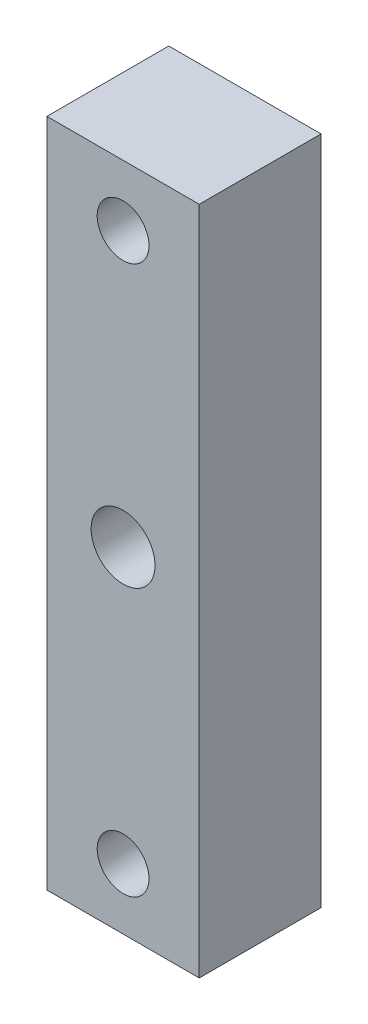
from build123d import *

# Parameters (mm, degrees)
SKETCH1_W                   = 25
SKETCH1_H                   = 110
BOSS_EXTRUDE1_DEPTH         = 20
SKETCH3_R                   = 4.25
CUT_EXTRUDE1_DEPTH          = 30
SKETCH5_R                   = 6.5
CUT_EXTRUDE3_DEPTH          = 10
M12X1_25_TAPPED_HOLE1_D     = 10.5
M12X1_25_TAPPED_HOLE1_DEPTH = 30.25
M12X1_25_TAPPED_HOLE1_TIP   = 3.15451825


with BuildPart() as part:
    # Sketch1 → Boss-Extrude1 (new body)
    with BuildSketch(Plane.XY):
        Rectangle(SKETCH1_W, SKETCH1_H)
    extrude(amount=BOSS_EXTRUDE1_DEPTH)

    # Sketch3 → Cut-Extrude1 (cut)
    with BuildSketch(Plane.XY.offset(20)):
        with Locations((0, 45)):
            Circle(SKETCH3_R)
        with Locations((0, -45)):
            Circle(SKETCH3_R)
    extrude(amount=-CUT_EXTRUDE1_DEPTH, mode=Mode.SUBTRACT)

    # Sketch5 → Cut-Extrude3 (cut)
    with BuildSketch(Plane(origin=(0, 0, 0), x_dir=(-1, 0, 0), z_dir=(0, 0, -1))):
        with Locations((0, 45)):
            Circle(SKETCH5_R)
        with Locations((0, -45)):
            Circle(SKETCH5_R)
    extrude(amount=-CUT_EXTRUDE3_DEPTH, mode=Mode.SUBTRACT)

    # M12x1.25 Tapped Hole1
    with Locations(Plane(origin=(0, 0, 0), x_dir=(-1, 0, 0), z_dir=(0, 0, -1))):
        with Locations((0, 0)):
            Hole(M12X1_25_TAPPED_HOLE1_D / 2, depth=M12X1_25_TAPPED_HOLE1_DEPTH)
            with Locations((0, 0, -(M12X1_25_TAPPED_HOLE1_DEPTH + M12X1_25_TAPPED_HOLE1_TIP / 2))):  # 118° drill point
                Cone(0, M12X1_25_TAPPED_HOLE1_D / 2, M12X1_25_TAPPED_HOLE1_TIP, mode=Mode.SUBTRACT)


solid = part.part
